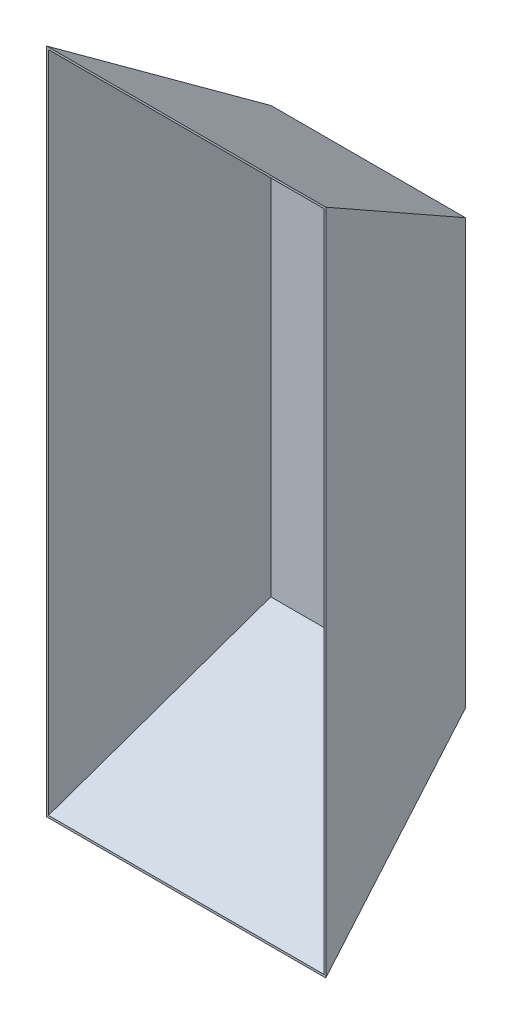
from build123d import *

# Parameters (mm, degrees)
SKETCH1_W           = 460
SKETCH1_H           = 1100
BOSS_EXTRUDE1_DEPTH = 300
CUT_EXTRUDE1_DEPTH  = 778.238702073
CUT_EXTRUDE3_DEPTH  = 949
SHELL1_T            = -3


with BuildPart() as part:
    # Sketch1 → Boss-Extrude1 (new body)
    with BuildSketch(Plane.XY):
        Rectangle(SKETCH1_W, SKETCH1_H)
    extrude(amount=-BOSS_EXTRUDE1_DEPTH)

    # Sketch3 → Cut-Extrude1 (cut, through all)
    with BuildSketch(Plane(origin=(230, 0, 0), x_dir=(0, 0, -1), z_dir=(1, 0, 0))):
        Polygon((0, 550), (300, 350), (300, 550), align=None)
        Polygon((300, -550), (0, -550), (300, -350), align=None)
    extrude(amount=-CUT_EXTRUDE1_DEPTH, mode=Mode.SUBTRACT)

    # Sketch6 → Cut-Extrude3 (cut, symmetric)
    with BuildSketch(Plane(origin=(0, 0, 0), x_dir=(1, 0, 0), z_dir=(0, 1, 0))):
        Polygon((-230, 0), (-160, 300), (-230, 300), align=None)
        Polygon((230, 300), (230, 0), (160, 300), align=None)
    extrude(amount=CUT_EXTRUDE3_DEPTH, both=True, mode=Mode.SUBTRACT)

    # Shell1
    shell1_openings = [part.faces().sort_by_distance(p)[0] for p in [
        (0, 0, 0),
    ]]
    offset(amount=SHELL1_T, openings=shell1_openings, kind=Kind.INTERSECTION)


solid = part.part
